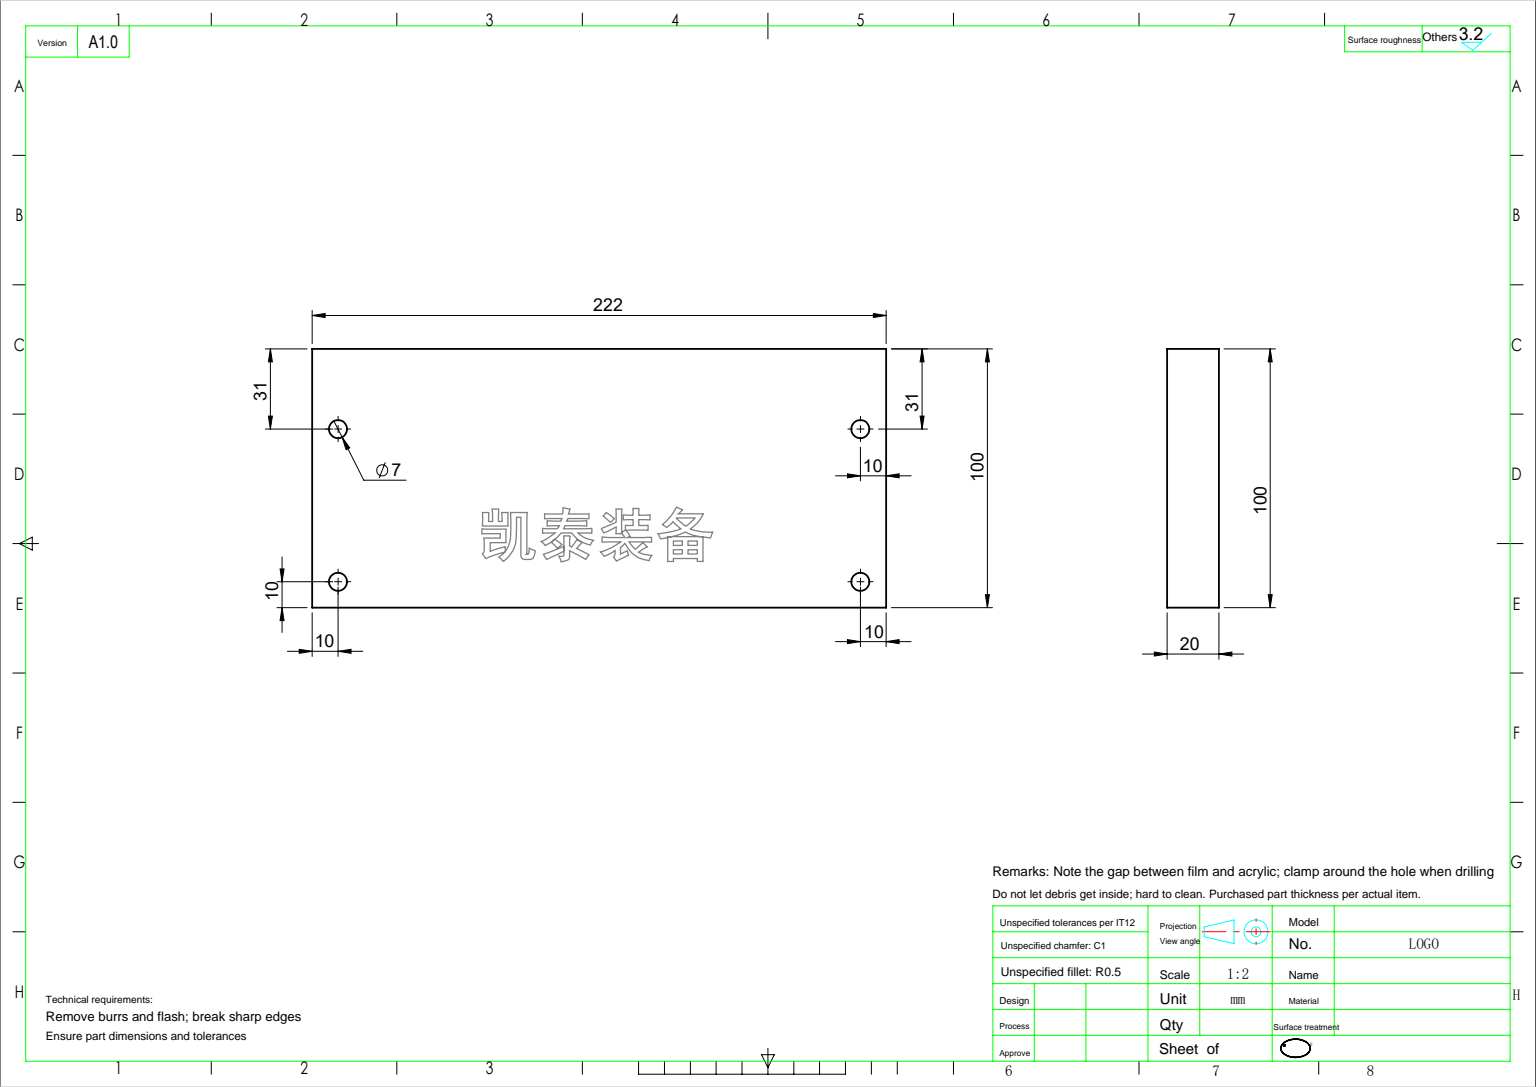
SolidWorks part; units mm, degrees
ref_plane "前视基准面" through (0, 0, 0) normal (0, 0, 1) x (1, 0, 0)
ref_plane "上视基准面" through (0, 0, 0) normal (0, 1, 0) x (1, 0, 0)
ref_plane "右视基准面" through (0, 0, 0) normal (1, 0, 0) x (0, 0, -1)
sketch "草图1" plane through (0, 0, 0) normal (0, 0, 1) x (1, 0, 0)
  line L1 (-111, 50) -> (111, 50)
  line L2 (-111, 50) -> (-111, -50)
  line L3 (-111, -50) -> (111, -50)
  line L4 (111, 50) -> (111, -50)
  line L5 (-111, 50) -> (111, -50) construction
  line L6 (-111, -50) -> (111, 50) construction
  point P0 (0, 0)
  dimension "D1" = 222
  dimension "D2" = 100
extrude "凸台-拉伸1" add sketch "草图1" along normal blind 20
sketch "草图2" plane through (0, 0, 20) normal (0, 0, 1) x (1, 0, 0)
  line L0 (-70, -30) -> (70, -30)
  line L3 (-111, -50) -> (111, -50) construction
  dimension "D1" = 20
sketch "草图3" plane through (0, 0, 20) normal (0, 0, 1) x (1, 0, 0)
  text T0 "<b>  凯泰装备</b>" font "黑体" height in points 50
sketch "草图4" plane through (0, 0, 20) normal (0, 0, 1) x (1, 0, 0)
  line L0 (-111, -50) -> (111, -50) construction
  line L1 (-111, 50) -> (-111, -50) construction
  line L2 (111, -50) -> (111, 50) construction
  line L3 (111, 50) -> (-111, 50) construction
  circle A0 centre (-101, 19) radius 3.5
  circle A1 centre (-101, -40) radius 3.5
  circle A2 centre (101, 19) radius 3.5
  circle A3 centre (101, -40) radius 3.5
  point P12 (0, 0)
  point P13 (0, 0)
  point P14 (0, 0)
  point P15 (0, 0)
  dimension "D1" = 7
  dimension "D3" = 10
  dimension "D4" = 10
  dimension "D2" = 10
  dimension "D5" = 31
extrude "切除-拉伸1" cut sketch "草图4" against normal through all
